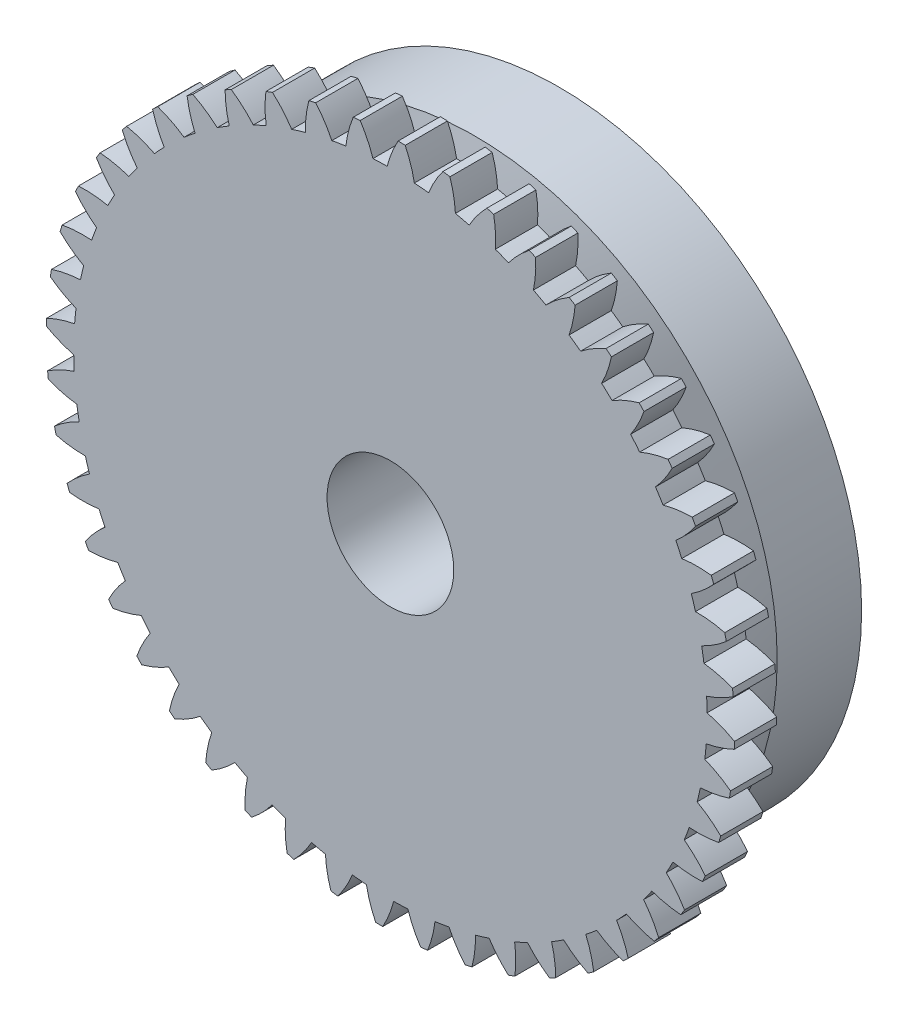
SolidWorks part; units mm, degrees
ref_plane "Front Plane" through (0, 0, 0) normal (0, 0, 1) x (1, 0, 0)
ref_plane "Top Plane" through (0, 0, 0) normal (0, 1, 0) x (1, 0, 0)
ref_plane "Right Plane" through (0, 0, 0) normal (1, 0, 0) x (0, 0, -1)
sketch "Sketch1" plane through (0, 0, 0) normal (0, 0, 1) x (1, 0, 0)
  circle A0 centre (0, 0) radius 7.16
  dimension "D1" = 14.32
extrude "Boss-Extrude1" add sketch "Sketch1" along normal blind 2
ref_plane "Plane1" through (0, 0, 3) normal (0, 0, 1) x (1, 0, 0)
sketch "Sketch2" plane through (0, 0, 3) normal (0, 0, 1) x (1, 0, 0)
  circle A0 centre (0, 0) radius 7.5
  dimension "D1" = 15
sketch "Sketch3" plane through (0, 0, 2) normal (0, 0, 1) x (1, 0, 0)
  circle A0 centre (0, 0) radius 7.16
loft "Loft3" add profiles "Sketch3", "Sketch2"
sketch "Sketch4" plane through (0, 0, 3) normal (0, 0, 1) x (1, 0, 0)
  circle A0 centre (0, 0) radius 7.5
  dimension "D1" = 15
extrude "Boss-Extrude2" add sketch "Sketch4" along normal blind 1
sketch "Sketch6" plane through (0, 0, 4) normal (0, 0, 1) x (1, 0, 0)
  line L0 (0, 0) -> (0, 9.4673) construction
  line L1 (0, 0) -> (0.3122, 9.5374) construction
  line L2 (0, 0) -> (3.4258, 9.4122) construction
  line L3 (0, 7.75) -> (2.4908, 6.8434) construction
  circle A1 centre (0, 0) radius 8.15 construction
  circle A2 centre (0, 0) radius 7.75 construction
  arc A3 (0.1834, 8.1479) -> (-0.0774, 7.4996) centre (2.4908, 6.8434) ccw
  arc A4 (0.5677, 7.4785) -> (-0.0774, 7.4996) centre (0, 0) ccw
  arc A6 (0.3499, 8.1425) -> (0.5677, 7.4785) centre (-2.0379, 6.9917) cw
  arc A7 (0.3499, 8.1425) -> (0, 8.15) centre (0, 0) ccw
  circle M10 centre (0, 0) radius 7.5
  dimension "D1" = 16.3
  dimension "D2" = 15.5
  dimension "D3" = 20
  dimension "D4" = 1.875
extrude "Boss-Extrude3" add sketch "Sketch6" against normal blind 1 contours A6 A7 A3 M10
pattern_circular "CirPattern1" count 48 over 360 about axis through (0, 0, 0) along (0, 0, 1) of "Boss-Extrude3"
sketch "Sketch7" plane through (0, 0, 4) normal (0, 0, 1) x (1, 0, 0)
  circle A0 centre (0, 0) radius 1.5
  dimension "D1" = 3
extrude "Cut-Extrude1" cut sketch "Sketch7" against normal blind 5
